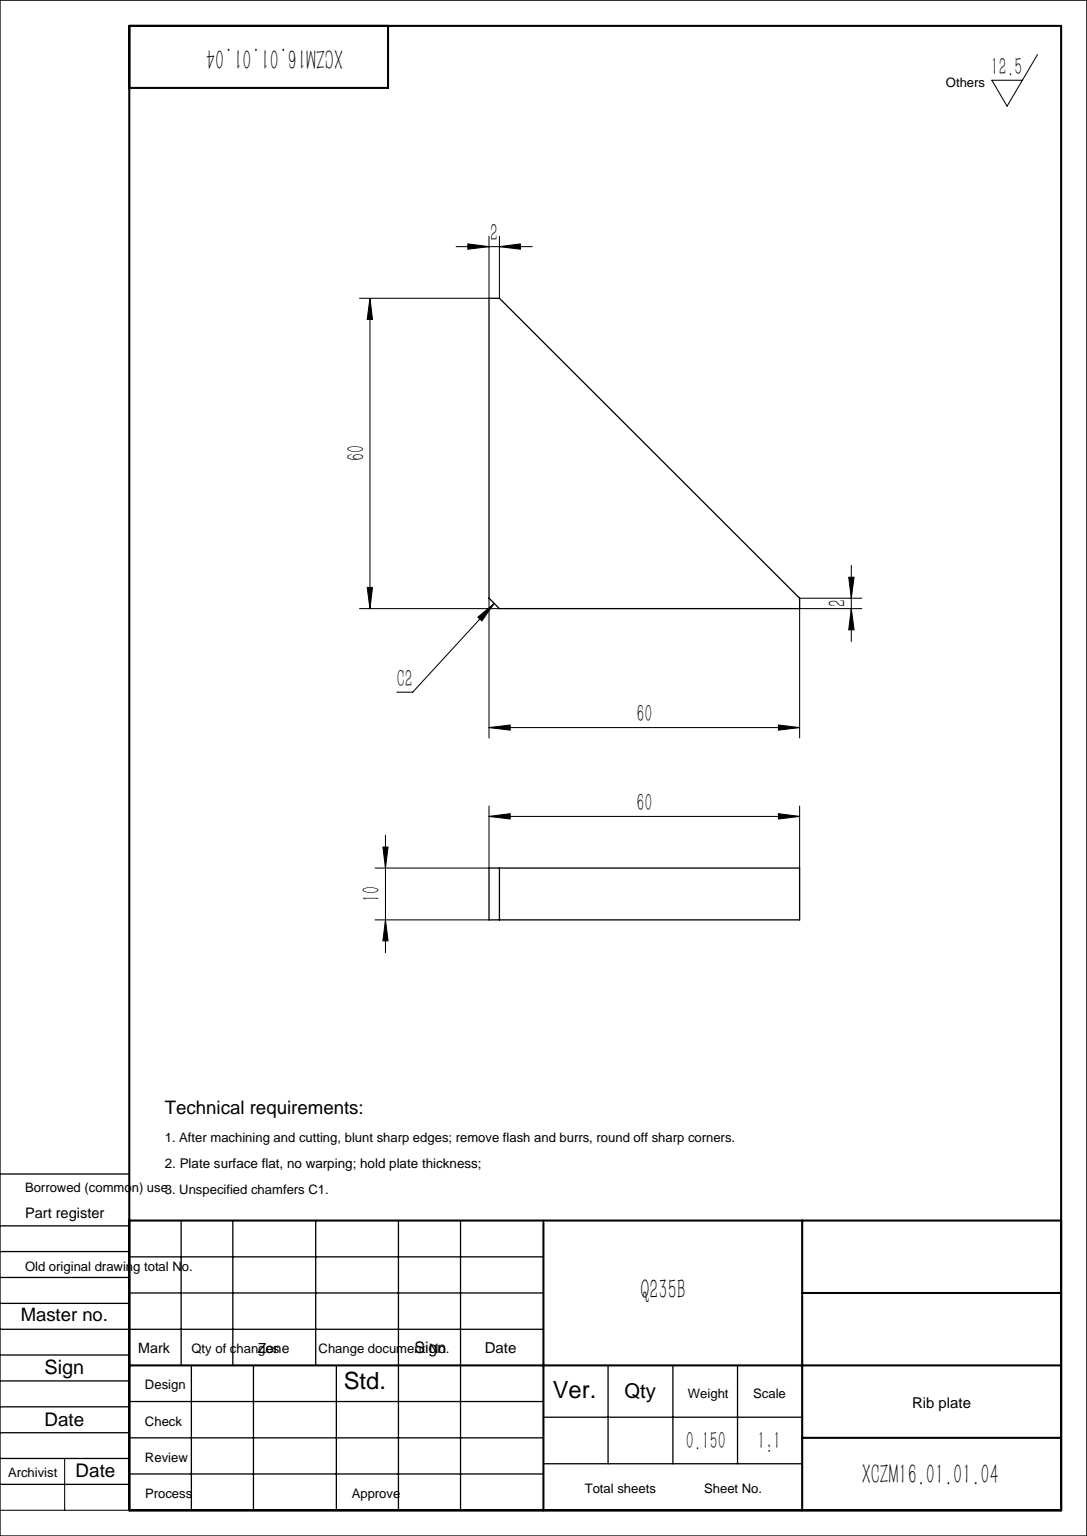
SolidWorks part; units mm, degrees
material "Q235B"
ref_plane "Front Plane" through (0, 0, 0) normal (0, 0, 1) x (1, 0, 0)
ref_plane "Top Plane" through (0, 0, 0) normal (0, 1, 0) x (1, 0, 0)
ref_plane "Right Plane" through (0, 0, 0) normal (1, 0, 0) x (0, 0, -1)
sketch "Sketch1" plane through (0, 0, 0) normal (0, 0, 1) x (1, 0, 0)
  line L0 (0, 60) -> (0, 0)
  line L1 (0, 0) -> (60, 0)
  line L2 (60, 0) -> (60, 2)
  line L3 (60, 2) -> (2, 60)
  line L4 (2, 60) -> (0, 60)
  dimension "D1" = 60
  dimension "D2" = 2
extrude "Boss-Extrude1" add sketch "Sketch1" along normal blind 10
chamfer "Chamfer1" distance 2 angle 45 1 edges at (0, 0, 5)
